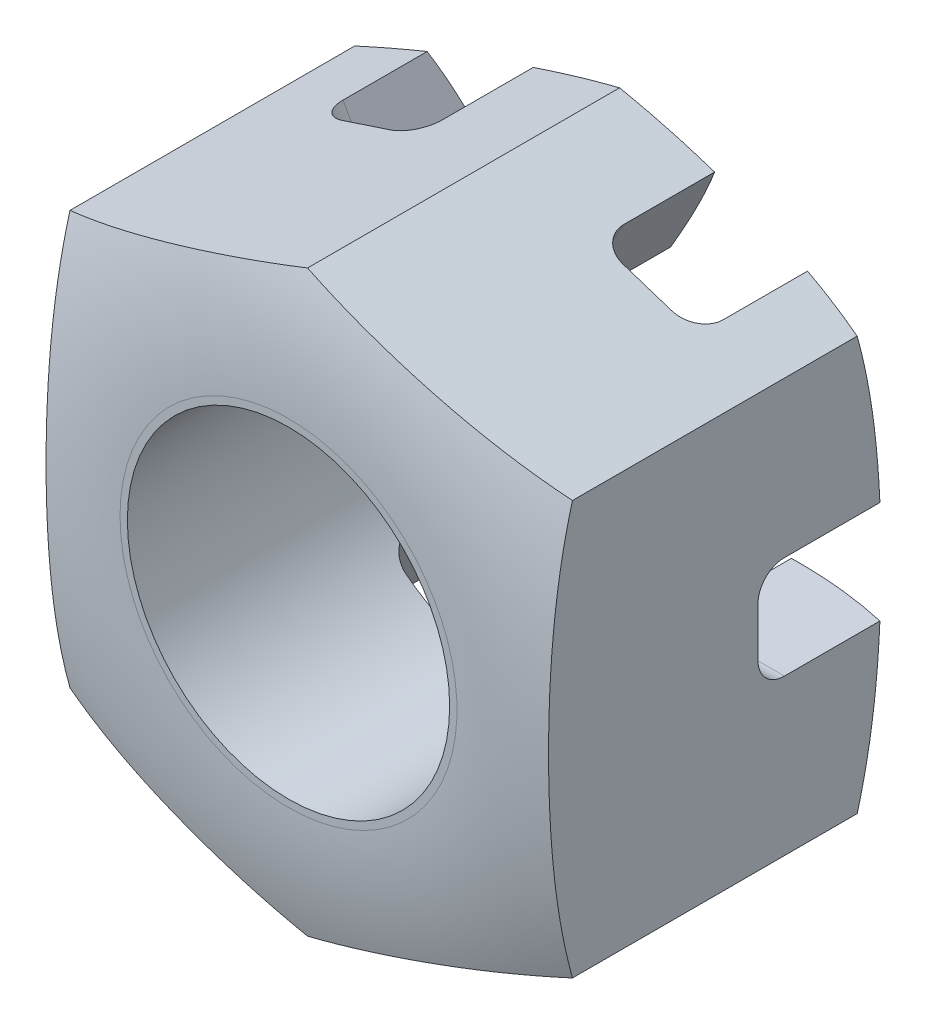
from build123d import *

# Parameters (mm, degrees)
BOSS_EXTRUDE1_DEPTH    = 23.9
SKETCH3_W              = 65
SKETCH3_H              = 7
CUT_EXTRUDE1_DEPTH     = 9
CIRPATTERN1_COUNT      = 3
CIRPATTERN1_ANGLE      = 120
M24X2_0_TAPPED_HOLE1_D = 22
FILLET2_R              = 1.8


with BuildPart() as part:
    # Sketch1 → Boss-Extrude1 (new body)
    with BuildSketch(Plane.XY):
        Polygon((0, 19.75), (-17.15, 14.1137269), (-17.15, -14.1137269), (0, -19.75), (17.15, -14.1137269), (17.15, 14.1137269), align=None)
    extrude(amount=BOSS_EXTRUDE1_DEPTH)

    # Sketch3 → Cut-Extrude1 (cut)
    with BuildSketch(Plane(origin=(0, 0, 0), x_dir=(-1, 0, 0), z_dir=(0, 0, -1))):
        Rectangle(SKETCH3_W, SKETCH3_H)
    cut_extrude1 = extrude(amount=-CUT_EXTRUDE1_DEPTH, mode=Mode.SUBTRACT)

    # CirPattern1: Cut-Extrude1 ×3 about axis
    cirpattern1_axis = Axis((0, 0, 0), (0, 0, 1))
    for i in range(1, CIRPATTERN1_COUNT):
        add(cut_extrude1.rotate(cirpattern1_axis, i * CIRPATTERN1_ANGLE / (CIRPATTERN1_COUNT - 1)), mode=Mode.SUBTRACT)

    # M24x2.0 Tapped Hole1 (through all)
    with Locations(Plane.XY.offset(23.9)):
        with Locations((0, 0)):
            Hole(M24X2_0_TAPPED_HOLE1_D / 2)

    # Fillet2
    fillet2_edges = [part.edges().sort_by_distance(p)[0] for p in [
        (-10.613150211, 11.382515394, 9),
        (4.185151513, 14.248895058, 9),
        (-4.185151513, -14.248895058, 9),
        (10.613150211, -11.382515394, 9),
        (-13.789163404, -3.5, 9),
        (13.789163404, 3.5, 9),
        (-13.789163404, 3.5, 9),
        (13.789163404, -3.5, 9),
        (-4.185151513, 14.248895058, 9),
        (4.185151513, -14.248895058, 9),
        (10.613150211, 11.382515394, 9),
        (-10.613150211, -11.382515394, 9),
    ]]
    fillet(fillet2_edges, radius=FILLET2_R)

    # Sketch8 → Cut-Revolve1 (revolve, cut)
    with BuildSketch(Plane(origin=(0, 0, 0), x_dir=(1, 0, 0), z_dir=(0, 1, 0))):
        with BuildLine():
            Line((11.5, 0), (33.520524336, 0))
            Line((33.520524336, 0), (33.520524336, -11.524643769))
            ThreePointArc((33.520524336, -11.524643769), (23.926995876, -3.055321154), (11.5, 0))
        make_face()
        with BuildLine():
            Line((11.5, -23.9), (28.830221364, -23.9))
            Line((28.830221364, -23.9), (28.830221364, -17.542686406))
            ThreePointArc((28.830221364, -17.542686406), (20.729734675, -22.260524594), (11.5, -23.9))
        make_face()
    revolve(axis=Axis((0, 0, -1.73), (0, 0, 1)), mode=Mode.SUBTRACT)


solid = part.part
